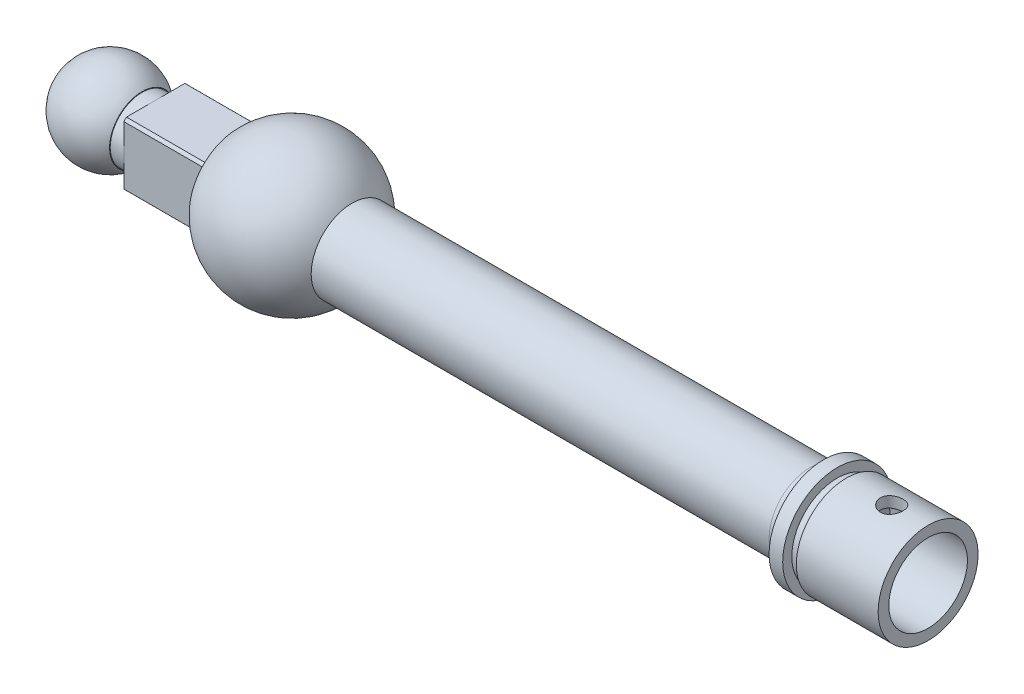
SolidWorks part; units mm, degrees
ref_plane "Front" through (0, 0, 0) normal (0, 0, 1) x (1, 0, 0)
ref_plane "Top" through (0, 0, 0) normal (0, 1, 0) x (1, 0, 0)
ref_plane "Right" through (0, 0, 0) normal (1, 0, 0) x (0, 0, -1)
sketch "Sketch1" plane through (0, 0, 0) normal (0, 0, 1) x (1, 0, 0)
  line L0 (62.3793, 22.2016) -> (258.035, 22.2016) construction
  line L1 (254.3793, 33.2016) -> (254.3793, 30.8516)
  line L2 (237.3793, 30.8516) -> (254.3793, 30.8516)
  line L3 (234.3793, 26.2016) -> (237.3793, 30.8516)
  line L4 (231.3793, 34.2016) -> (234.3793, 34.2016)
  line L5 (234.3793, 34.2016) -> (234.3793, 32.2016)
  line L6 (236.3793, 33.2016) -> (254.3793, 33.2016)
  line L7 (236.3793, 33.2016) -> (236.3793, 32.2016)
  line L8 (234.3793, 32.2016) -> (236.3793, 32.2016)
  line L9 (127.608, 31.2016) -> (228.3793, 31.2016)
  line L10 (81.3793, 29.2016) -> (84.3793, 29.2016)
  line L11 (66.3793, 28.2016) -> (66.3793, 26.2016)
  line L12 (66.3793, 26.2016) -> (172.6479, 26.2016)
  line L13 (172.6479, 26.2016) -> (234.3793, 26.2016)
  line L14 (84.3793, 31.7016) -> (102.3793, 31.7016)
  line L15 (84.3793, 31.7016) -> (84.3793, 29.2016)
  line L16 (81.3793, 29.343) -> (81.3793, 29.2016)
  line L17 (102.3793, 31.7016) -> (102.3793, 32.7846)
  arc A0 (127.608, 31.2016) -> (102.3793, 32.7846) centre (114.3793, 22.2016) ccw
  arc A1 (228.3793, 31.2016) -> (231.3793, 34.2016) centre (228.3793, 34.2016) ccw
  arc A2 (81.3793, 29.343) -> (66.3793, 28.2016) centre (74.3793, 22.2016) ccw
revolve "Revolve1" add sketch "Sketch1" angle 360 about L0
sketch "Sketch2" plane through (84.3793, 0, 0) normal (-1, 0, 0) x (0, 0, 1)
  line L1 (-7, 29.2016) -> (7, 29.2016)
  line L2 (-7, 29.2016) -> (-7, 15.2016)
  line L3 (-7, 15.2016) -> (7, 15.2016)
  line L4 (7, 29.2016) -> (7, 15.2016)
  line L5 (-7, 29.2016) -> (7, 15.2016) construction
  line L6 (-7, 15.2016) -> (7, 29.2016) construction
  circle A0 centre (0, 22.2016) radius 25.6925
  point P0 (0, 22.2016)
  dimension "D1" = 14
extrude "Cut-Extrude1" cut sketch "Sketch2" against normal up to surface (18 mm away) up to face at (102.3793, 22.2016, 9.5)
sketch "Sketch3" [suppressed] plane through (0, 0, 0) normal (0, 0, 1) x (1, 0, 0)
  line L0 (246.3793, 22.2016) -> (84.3793, 22.2016) construction
  line L1 (66.3793, 28.2016) -> (66.3793, 16.2016) construction
  circle A0 centre (246.3793, 22.2016) radius 2.5
  dimension "D2" = 5
  dimension "D1" = 180
sketch "Sketch4" plane through (0, 29.2016, 0) normal (0, 1, 0) x (1, 0, 0)
  line L0 (254.3793, -11) -> (254.3793, 11) construction
  circle A0 centre (246.3793, 0) radius 2.5
  dimension "D1" = 8
extrude "Cut-Extrude3" cut sketch "Sketch4" along normal blind 10 contours A0
